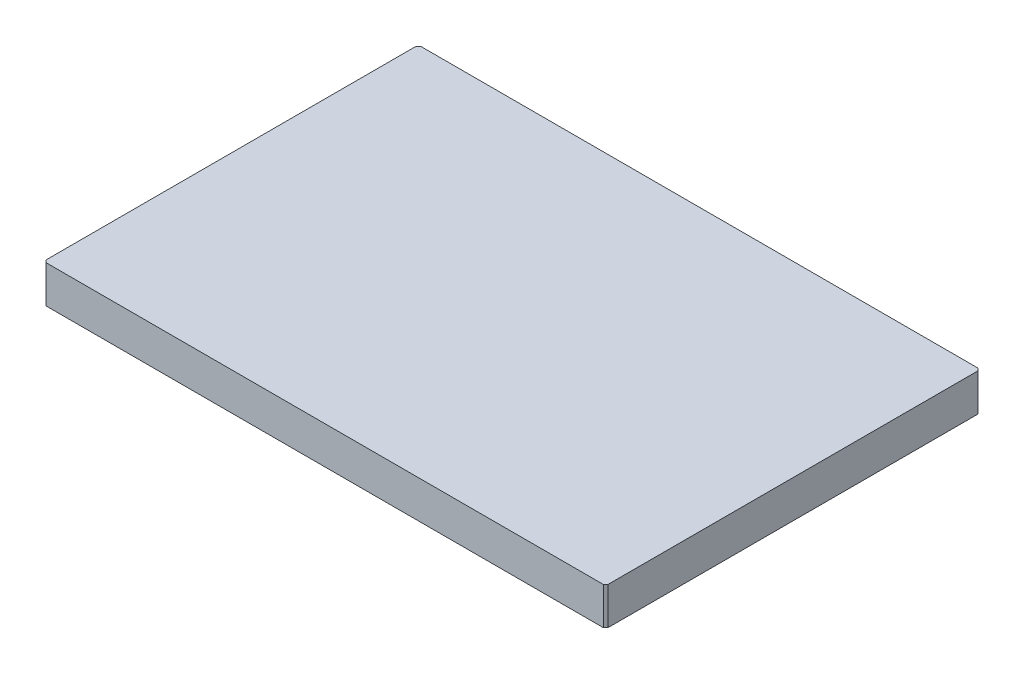
from build123d import *

# Parameters (mm, degrees)
SKETCH1_W              = 1200
SKETCH1_H              = 800
BOSS_EXTRUDE1_DEPTH    = 80
CHAMFER1_SIZE          = 5
M16_TAPPED_HOLE1_D     = 14
M16_TAPPED_HOLE1_DEPTH = 38
M16_TAPPED_HOLE1_TIP   = 4.206024333


with BuildPart() as part:
    # Sketch1 → Boss-Extrude1 (new body)
    with BuildSketch(Plane(origin=(0, 0, 0), x_dir=(1, 0, 0), z_dir=(0, 1, 0))):
        Rectangle(SKETCH1_W, SKETCH1_H)
    extrude(amount=BOSS_EXTRUDE1_DEPTH)

    # Chamfer1
    chamfer1_edges = [part.edges().sort_by_distance(p)[0] for p in [
        (600, 40, 400),
        (-600, 40, 400),
        (-600, 40, -400),
        (600, 40, -400),
    ]]
    chamfer(chamfer1_edges, length=CHAMFER1_SIZE)

    # M16 Tapped Hole1
    with Locations(Plane(origin=(0, 0, 0), x_dir=(-1, 0, 0), z_dir=(0, -1, 0))):
        with Locations((0, -200), (100, -173.205080757), (173.205080757, -100), (200, 0), (173.205080757, 100), (100, 173.205080757), (0, 200), (-100, 173.205080757), (-173.205080757, 100), (-200, 0), (-173.205080757, -100), (-100, -173.205080757)):
            Hole(M16_TAPPED_HOLE1_D / 2, depth=M16_TAPPED_HOLE1_DEPTH)
            with Locations((0, 0, -(M16_TAPPED_HOLE1_DEPTH + M16_TAPPED_HOLE1_TIP / 2))):  # 118° drill point
                Cone(0, M16_TAPPED_HOLE1_D / 2, M16_TAPPED_HOLE1_TIP, mode=Mode.SUBTRACT)


solid = part.part
